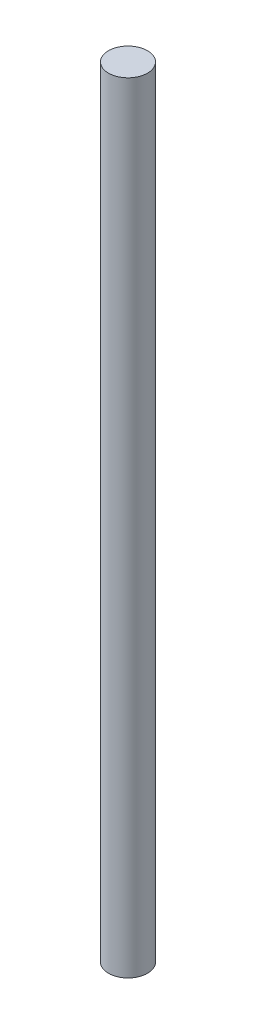
from build123d import *

# Parameters (mm, degrees)
SKETCH1_R           = 10
BOSS_EXTRUDE1_DEPTH = 400


with BuildPart() as part:
    # Sketch1 → Boss-Extrude1 (new body)
    with BuildSketch(Plane(origin=(0, 0, 0), x_dir=(1, 0, 0), z_dir=(0, 1, 0))):
        with Locations(Location((0, 0, 0), (0, 0, 270))):
            Circle(SKETCH1_R)
    extrude(amount=BOSS_EXTRUDE1_DEPTH)


solid = part.part
